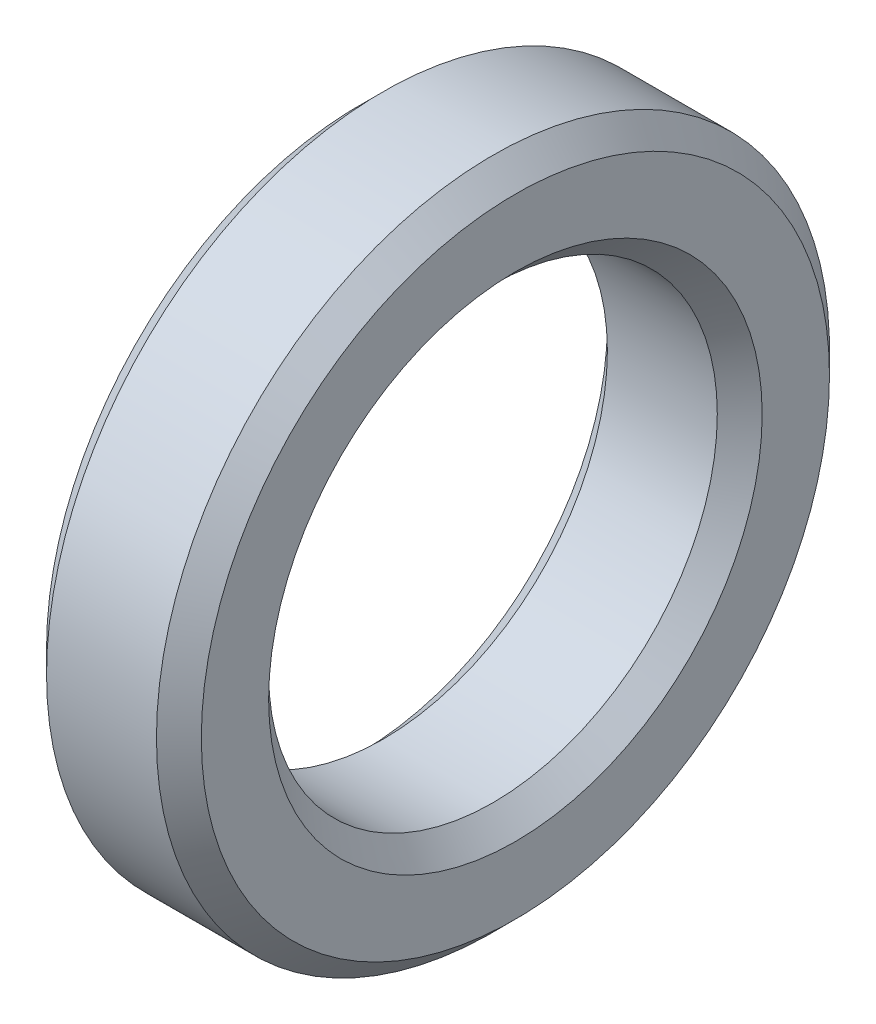
SolidWorks part; units mm, degrees
material "Q235B"
ref_plane "Front Plane" through (0, 0, 0) normal (0, 0, 1) x (1, 0, 0)
ref_plane "Top Plane" through (0, 0, 0) normal (0, 1, 0) x (1, 0, 0)
ref_plane "Right Plane" through (0, 0, 0) normal (1, 0, 0) x (0, 0, -1)
sketch "Sketch1" plane through (0, 0, 0) normal (1, 0, 0) x (0, 0, -1)
  circle A0 centre (0, 0) radius 10
  circle A1 centre (0, 0) radius 15
  dimension "D1" = 20
  dimension "D2" = 30
extrude "Boss-Extrude1" add sketch "Sketch1" along normal blind 6.9
chamfer "Chamfer1" distance 1 angle 45 4 edges at (0, 0, -15) (6.9, 0, -15) (0, 0, -10) (6.9, 0, -10)
